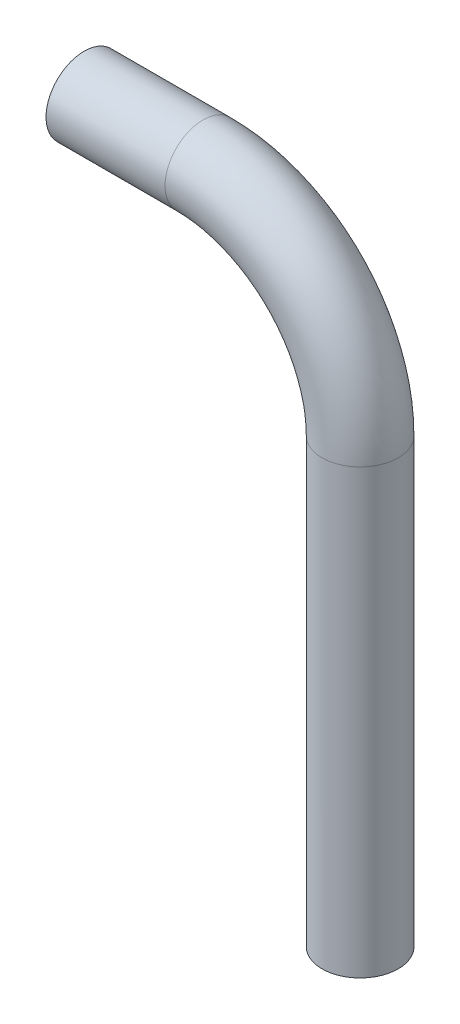
from build123d import *

# Parameters (mm, degrees)
SKETCH2_R = 4


with BuildPart() as part:
    # Sweep1: sweep along a path in Sketch1
    with BuildLine(Plane.XY) as sweep1_path:
        Line((0, 0), (12.5, 0))
        ThreePointArc((12.5, 0), (24.16726189, -4.83273811), (29, -16.5))
        Line((29, -16.5), (29, -63))
    # Sketch2 → Sweep1 (sweep)
    with BuildSketch(Plane(origin=(0, 0, 0), x_dir=(0, 0, -1), z_dir=(1, 0, 0))):
        Circle(SKETCH2_R)
    sweep(path=sweep1_path.line)


solid = part.part
